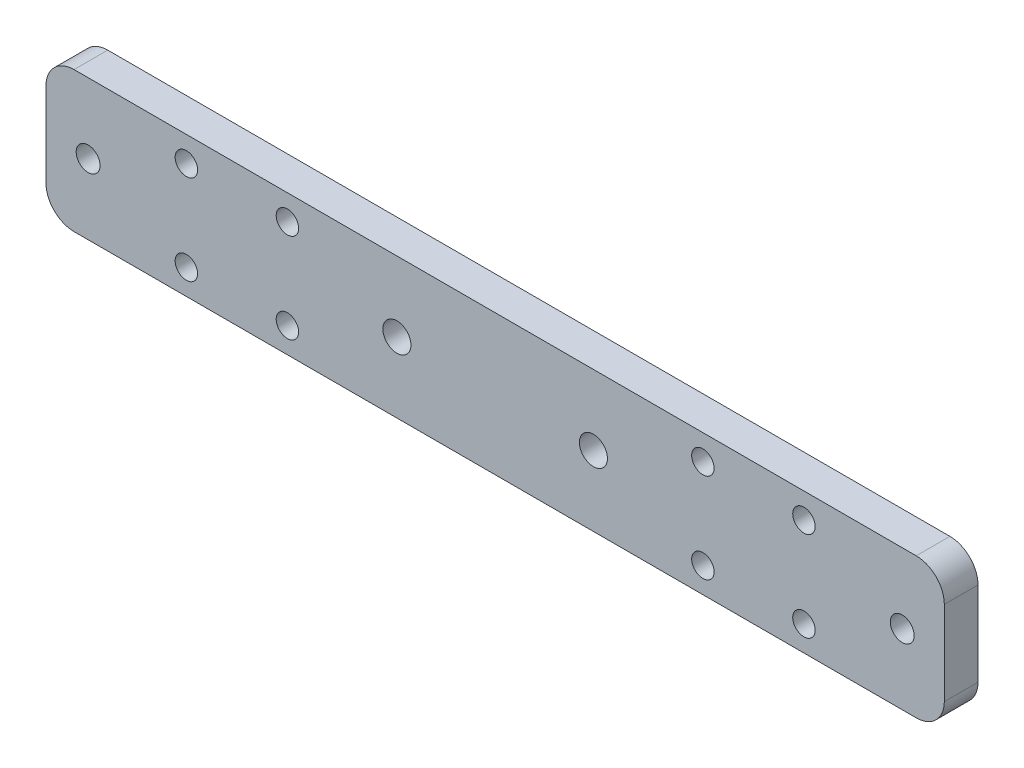
SolidWorks part; units mm, degrees
material "普通碳钢"
ref_plane "Front Plane" through (0, 0, 0) normal (0, 0, 1) x (1, 0, 0)
ref_plane "Top Plane" through (0, 0, 0) normal (0, 1, 0) x (1, 0, 0)
ref_plane "Right Plane" through (0, 0, 0) normal (1, 0, 0) x (0, 0, -1)
sketch "Sketch1" plane through (0, 0, 0) normal (0, 0, 1) x (1, 0, 0)
  line L0 (0, 0) -> (320, 0)
  line L1 (160, 50) -> (160, 45.2964) construction
  line L2 (320, 0) -> (320, 50)
  line L3 (320, 50) -> (0, 50)
  line L4 (0, 0) -> (0, 50)
  circle A0 centre (50, 41) radius 4
  circle A1 centre (86, 41) radius 4
  circle A2 centre (86, 9) radius 4
  circle A3 centre (50, 9) radius 4
  circle A4 centre (270, 9) radius 4
  circle A5 centre (234, 9) radius 4
  circle A6 centre (234, 41) radius 4
  circle A7 centre (270, 41) radius 4
  circle A8 centre (125, 25) radius 5
  circle A9 centre (195, 25) radius 5
  dimension "D3" = 8
  dimension "D11" = 10
  dimension "D7" = 9
  dimension "D9" = 25
  dimension "D1" = 320
  dimension "D2" = 50
  dimension "D4" = 32
  dimension "D5" = 36
  dimension "D6" = 70
  dimension "D8" = 50
extrude "Boss-Extrude1" add sketch "Sketch1" along normal blind 12
hole_wizard "M10 Tapped Hole1" positions "Sketch4" profile "Sketch5" tap size "M10" standard "GB"
sketch "Sketch4" plane through (0, 0, 12) normal (0, 0, 1) x (1, 0, 0)
  line L0 (50, 41) -> (50, 9) construction
  line L2 (15, 25) -> (50, 25) construction
  circle A0 centre (270, 9) radius 4 construction
  point P0 (15, 25)
  point P13 (305, 25)
  dimension "D2" = 35
  dimension "D1" = 35
sketch "Sketch5" plane through (15, 25, 12) normal (1, 0, 0) x (0, -1, 0)
  line L0 (0, 0) -> (0, 27.0537)
  line L1 (0, 27.0537) -> (4.25, 24.5)
  line L2 (4.25, 24.5) -> (4.25, 0)
  line L5 (4.25, 0) -> (0, 0)
  line L10 (0, 27.0537) -> (-4.25, 24.5) construction
  line L11 (0, -6.35) -> (0, 107.95) construction
  dimension "螺纹孔钻头直径" = 8.5
  dimension "螺纹孔钻头深度" = 24.5
  dimension "导头角度" = 118
cosmetic thread "Hole Cosmetic Thread2" parameters "D1"=20, "D2"=9.5
cosmetic thread "Hole Cosmetic Thread3" parameters "D1"=20, "D2"=9.5
fillet "Fillet1" radius 10 4 edges at (320, 50, 6) (320, 0, 6) (0, 50, 6) (0, 0, 6)
